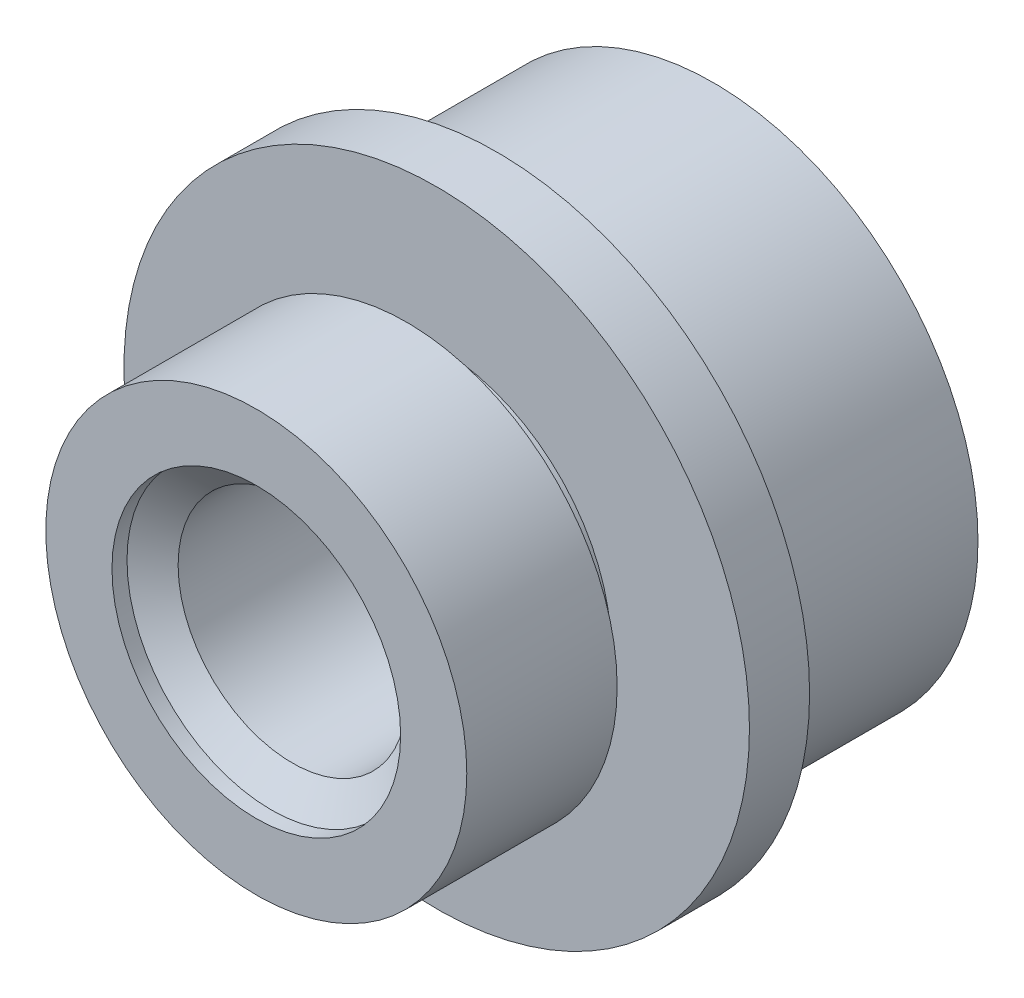
from build123d import *


with BuildPart() as part:
    # Sketch2 → Revolve1 (revolve)
    with BuildSketch(Plane(origin=(0, 0, 0), x_dir=(0, 0, -1), z_dir=(1, 0, 0)), mode=Mode.PRIVATE) as revolve1_sk:
        Polygon((0, 17.5), (0, 12), (1.25, 12), (3.000518846, 9.5), (23, 9.5), (38, 14), (38, 22), (20, 22), (20, 26), (15, 26), (15, 14.5), (12.5, 14.5), (12.5, 17.5), align=None)
    revolve(revolve1_sk.sketch.rotate(Axis((0, 0, 28.492460363), (0, 0, -1)), 90), axis=Axis((0, 0, 28.492460363), (0, 0, -1)))


solid = part.part
